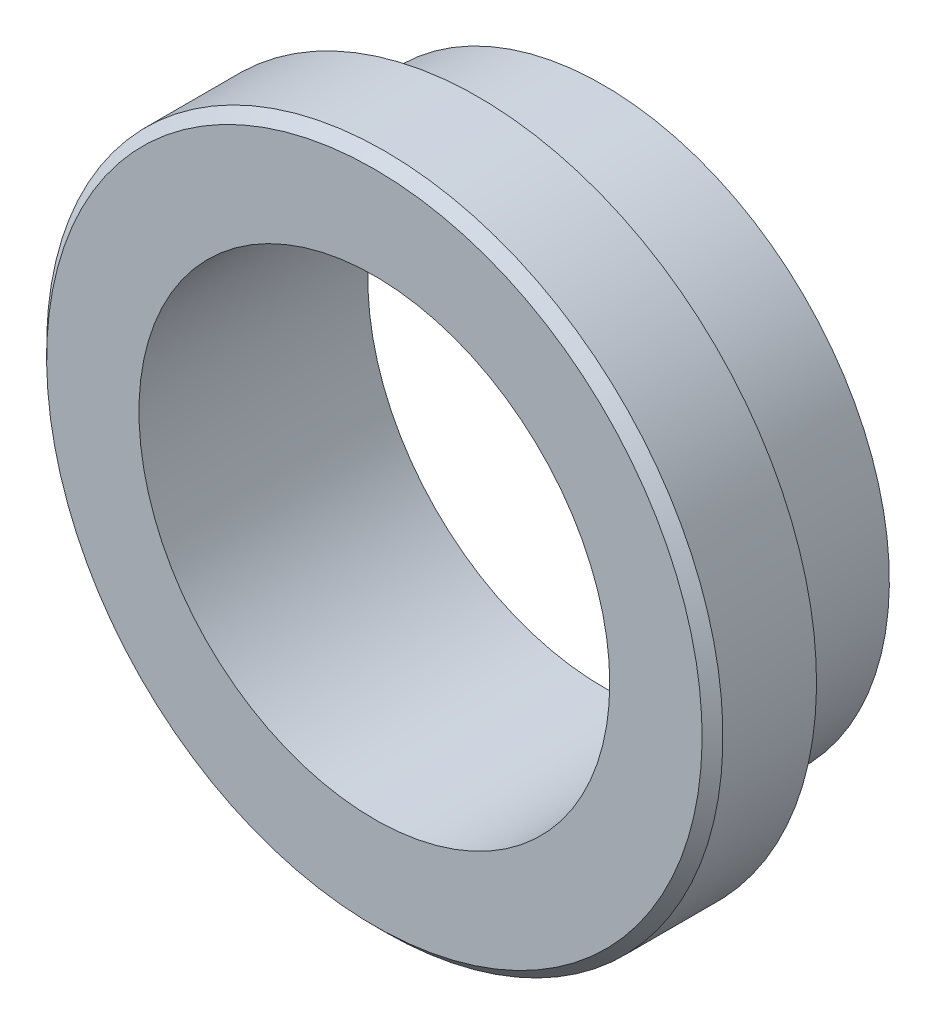
SolidWorks part; units mm, degrees
material "45#调质"
ref_plane "Front Plane" through (0, 0, 0) normal (0, 0, 1) x (1, 0, 0)
ref_plane "Top Plane" through (0, 0, 0) normal (0, 1, 0) x (1, 0, 0)
ref_plane "Right Plane" through (0, 0, 0) normal (1, 0, 0) x (0, 0, -1)
sketch "Sketch1" plane through (0, 0, 0) normal (1, 0, 0) x (0, 0, -1)
  line L0 (0, 0) -> (0, 27.5)
  line L1 (0, 27.5) -> (-12, 27.5)
  line L2 (-12, 27.5) -> (-12, 32.5)
  line L3 (-12, 32.5) -> (-22, 32.5)
  line L4 (-22, 32.5) -> (-22, 0)
  line L5 (-22, 0) -> (0, 0)
  dimension "D1" = 27.5
  dimension "D2" = 5
  dimension "D3" = 12
  dimension "D4" = 10
revolve "Revolve1" add sketch "Sketch1" angle 360 about L5
hole_wizard "G1-1/2 Tapped Hole1" positions "Sketch2" profile "Sketch3" tap size "G1-1/2" standard "GB" end condition through all
sketch "Sketch2" plane through (0, 0, 22) normal (0, 0, 1) x (1, 0, 0)
  point P0 (0, 0)
sketch "Sketch3" plane through (0, 0, 22) normal (1, 0, 0) x (0, -1, 0)
  line L0 (0, 0) -> (0, 22)
  line L1 (0, 22) -> (22.625, 22)
  line L2 (22.625, 22) -> (22.625, 0)
  line L5 (22.625, 0) -> (0, 0)
  line L11 (0, -6.35) -> (0, 107.95) construction
  dimension "通孔螺纹孔钻头直径" = 45.25
  dimension "通孔螺纹孔钻头深度" = 22
cosmetic thread "Cosmetic thread1" parameters "D2"=47.803
chamfer "Chamfer1" distance 1 angle 45 1 edges at (0, -32.5, 22)
